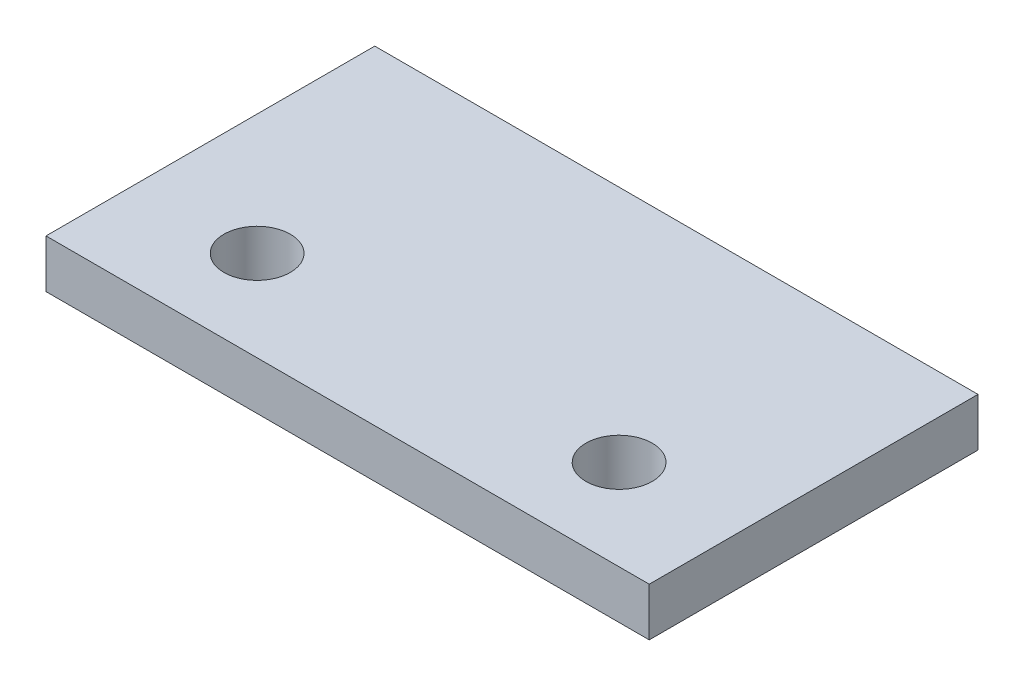
SolidWorks part; units mm, degrees
material "Q235B"
ref_plane "Front Plane" through (0, 0, 0) normal (0, 0, 1) x (1, 0, 0)
ref_plane "Top Plane" through (0, 0, 0) normal (0, 1, 0) x (1, 0, 0)
ref_plane "Right Plane" through (0, 0, 0) normal (1, 0, 0) x (0, 0, -1)
sketch "Sketch1" plane through (0, 0, 0) normal (0, 1, 0) x (1, 0, 0)
  line L1 (50, -27.25) -> (-50, -27.25)
  line L2 (50, -27.25) -> (50, 27.25)
  line L3 (50, 27.25) -> (-50, 27.25)
  line L4 (-50, -27.25) -> (-50, 27.25)
  line L5 (50, -27.25) -> (-50, 27.25) construction
  line L6 (50, 27.25) -> (-50, -27.25) construction
  point P0 (0, 0)
  dimension "D1" = 54.5
  dimension "D2" = 100
extrude "Boss-Extrude1" add sketch "Sketch1" along normal blind 8
hole_wizard "Ø11.0 (11) Diameter Hole1" positions "Sketch2" profile "Sketch3" hole size "Ø11.0" standard "GB" end condition up to next
sketch "Sketch2" plane through (0, 8, 0) normal (0, 1, 0) x (1, 0, 0)
  line L0 (0, -12.25) -> (-30, -12.25) construction
  line L2 (0, -12.25) -> (0, 27.25) construction
  line L3 (50, 27.25) -> (-50, 27.25) construction
  line L5 (-50, -27.25) -> (50, -27.25) construction
  point P0 (-30, -12.25)
  point P13 (30, -12.25)
  dimension "D1" = 60
  dimension "D2" = 15
sketch "Sketch3" plane through (-30, 8, 12.25) normal (1, 0, 0) x (0, 0, 1)
  line L0 (0, 0) -> (0, 8)
  line L1 (0, 8) -> (5.5, 8)
  line L2 (5.5, 8) -> (5.5, 0)
  line L5 (5.5, 0) -> (0, 0)
  line L11 (0, -6.35) -> (0, 107.95) construction
  dimension "通孔孔直径" = 11
  dimension "通孔孔深度" = 8
